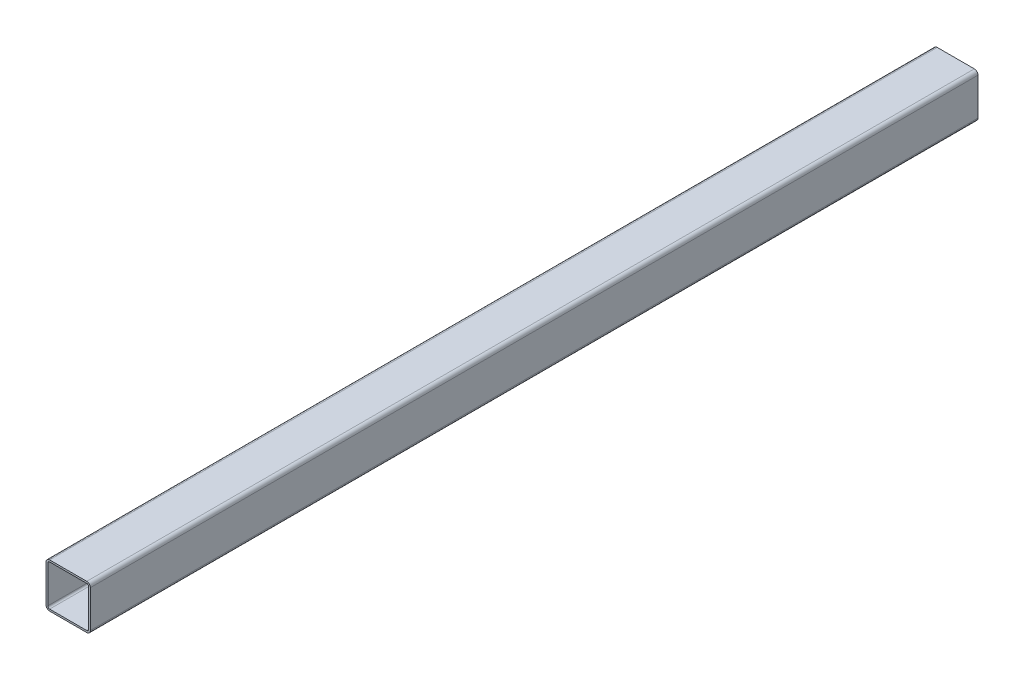
from build123d import *

# Parameters (mm, degrees)
BOSS_EXTRUDE1_DEPTH = 2000
SHELL1_T            = -4


with BuildPart() as part:
    # Sketch1 → Boss-Extrude1 (new body)
    with BuildSketch(Plane.XY):
        with BuildLine():
            Line((41.8, 50), (-41.8, 50))
            ThreePointArc((-41.8, 50), (-47.598275606, 47.598275606), (-50, 41.8))
            Line((-50, 41.8), (-50, -41.8))
            ThreePointArc((-50, -41.8), (-47.598275606, -47.598275606), (-41.8, -50))
            Line((-41.8, -50), (41.8, -50))
            ThreePointArc((41.8, -50), (47.598275606, -47.598275606), (50, -41.8))
            Line((50, -41.8), (50, 41.8))
            ThreePointArc((50, 41.8), (47.598275606, 47.598275606), (41.8, 50))
        make_face()
    extrude(amount=BOSS_EXTRUDE1_DEPTH)

    # Shell1
    shell1_openings = [part.faces().sort_by_distance(p)[0] for p in [
        (0, 0, 2000),
        (0, 0, 0),
    ]]
    offset(amount=SHELL1_T, openings=shell1_openings, kind=Kind.INTERSECTION)


solid = part.part
